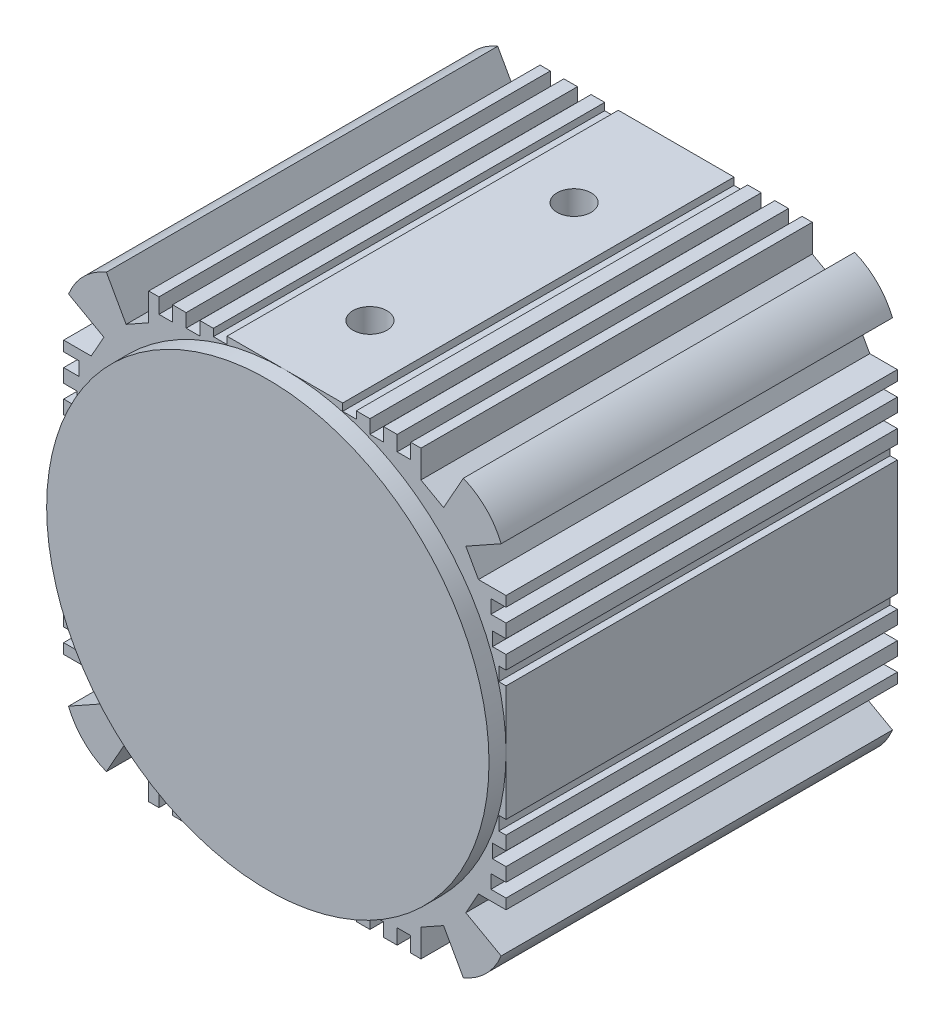
SolidWorks part; units mm, degrees
ref_plane "Front Plane" through (0, 0, 0) normal (0, 0, 1) x (1, 0, 0)
ref_plane "Top Plane" through (0, 0, 0) normal (0, 1, 0) x (1, 0, 0)
ref_plane "Right Plane" through (0, 0, 0) normal (1, 0, 0) x (0, 0, -1)
sketch "Sketch2" plane through (0, 0, 0) normal (0, 0, 1) x (1, 0, 0)
  line L1 (-65, -65) -> (65, -65)
  line L2 (-65, -65) -> (-65, 65)
  line L3 (-65, 65) -> (65, 65)
  line L4 (65, -65) -> (65, 65)
  line L5 (0, 65) -> (0, -65) construction
  line L6 (-65, 0) -> (65, 0) construction
  point P0 (0, 0)
  dimension "D1" = 130
  dimension "D2" = 130
extrude "Boss-Extrude2" add sketch "Sketch2" along normal blind 120
sketch "Sketch3" plane through (0, 0, 120) normal (0, 0, 1) x (1, 0, 0)
  circle A0 centre (0, 0) radius 65
  circle A1 centre (0, 0) radius 110.5255
  dimension "D1" = 130
extrude "Cut-Extrude1" cut sketch "Sketch3" against normal blind 5
fillet "Fillet1" radius 20 4 edges at (-65, -65, 57.5) (65, -65, 57.5) (-65, 65, 57.5) (65, 65, 57.5)
sketch "Sketch4" plane through (0, 0, 115) normal (0, 0, 1) x (1, 0, 0)
  line L0 (-55.1228, 68.3439) -> (-46.6441, 53.1849)
  line L1 (-46.6441, 53.1849) -> (-40, 56.9011)
  line L2 (-40, 56.9011) -> (-40, 68.3439)
  line L3 (-40, 68.3439) -> (-55.1228, 68.3439)
  line L5 (-37, 76.1289) -> (-33, 76.1289)
  line L6 (-37, 76.1289) -> (-37, 60.5589)
  line L7 (-37, 60.5589) -> (-33, 60.5589)
  line L8 (-33, 76.1289) -> (-33, 60.5589)
  line L9 (-35, 60.5589) -> (-35, 76.1289) construction
  line L10 (-37, 68.3439) -> (-33, 68.3439) construction
  line L11 (-29, 84.4734) -> (-25, 84.4734)
  line L12 (-29, 84.4734) -> (-29, 61.0315)
  line L13 (-29, 61.0315) -> (-25, 61.0315)
  line L14 (-25, 84.4734) -> (-25, 61.0315)
  line L15 (-27, 61.0315) -> (-27, 84.4734) construction
  line L16 (-29, 72.7525) -> (-25, 72.7525) construction
  line L17 (-21, 85.2411) -> (-17, 85.2411)
  line L18 (-21, 85.2411) -> (-21, 62.8725)
  line L19 (-21, 62.8725) -> (-17, 62.8725)
  line L20 (-17, 85.2411) -> (-17, 62.8725)
  line L21 (-19, 62.8725) -> (-19, 85.2411) construction
  line L22 (-21, 74.0568) -> (-17, 74.0568) construction
  point P4 (-35, 68.3439)
  point P6 (-27, 72.7525)
  point P12 (-19, 74.0568)
  dimension "D1" = 4
  dimension "D2" = 4
  dimension "D3" = 4
  dimension "D4" = 4
  dimension "D5" = 4
  dimension "D6" = 3
  dimension "D7" = 17
extrude "Cut-Extrude2" cut sketch "Sketch4" against normal blind 200
mirror "Mirror1" about plane through (0, 0, 0) normal (1, 0, 0) of "Cut-Extrude2"
pattern_circular "CirPattern2" count 4 every 90 about axis through (0, 0, 0) along (0, 0, 1) of "Cut-Extrude2", "Mirror1"
sketch "Sketch5" plane through (0, 65, 0) normal (0, 1, 0) x (1, 0, 0)
  line L0 (17, 0) -> (-17, 0) construction
  circle A0 centre (0, -90) radius 5
  circle A1 centre (0, -30) radius 5
  dimension "D1" = 30
  dimension "D2" = 60
extrude "Cut-Extrude3" cut sketch "Sketch5" against normal blind 10
